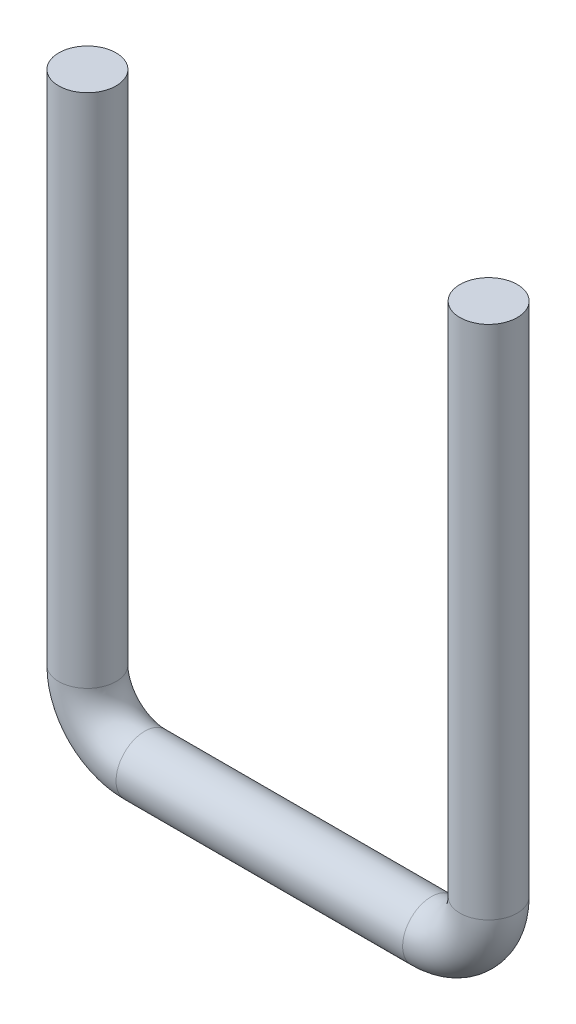
from build123d import *

# Parameters (mm, degrees)
SWEEP1_PROFILE_R = 5


with BuildPart() as part:
    # Sweep1: sweep along a path in Sketch1
    with BuildLine(Plane.XY) as sweep1_path:
        Line((-35, 100), (-35, 10))
        ThreePointArc((-35, 10), (-32.071067812, 2.928932188), (-25, 0))
        Line((-25, 0), (25, 0))
        ThreePointArc((25, 0), (32.071067812, 2.928932188), (35, 10))
        Line((35, 10), (35, 100))
    # Sweep1 profile (on start of the path) → Sweep1 (sweep)
    with BuildSketch(Plane(origin=(-35, 100, 0), x_dir=(0, 0, -1), z_dir=(0, -1, 0))):
        Circle(SWEEP1_PROFILE_R)
    sweep(path=sweep1_path.line)


solid = part.part
